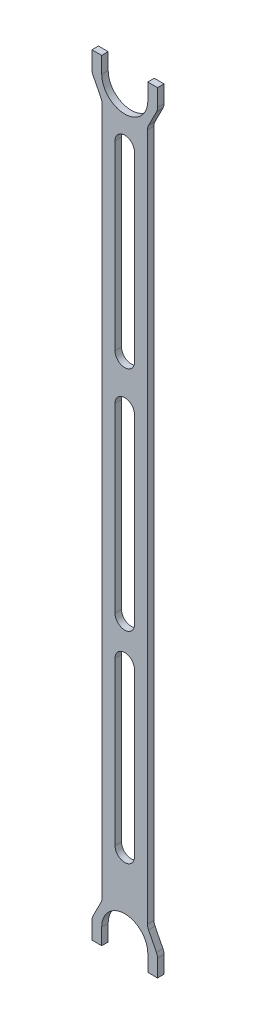
SolidWorks part; units mm, degrees
material "Thornel Mat VMA"
ref_plane "前视基准面" through (0, 0, 0) normal (0, 0, 1) x (1, 0, 0)
ref_plane "上视基准面" through (0, 0, 0) normal (0, 1, 0) x (1, 0, 0)
ref_plane "右视基准面" through (0, 0, 0) normal (1, 0, 0) x (0, 0, -1)
other "Configuration Table"
sketch "草图1" plane through (0, 0, 0) normal (0, 0, 1) x (1, 0, 0)
  line L0 (0, 106.65) -> (0, -106.65) construction
  line L1 (-7, 106.65) -> (-7, -106.65)
  line L2 (7, 106.65) -> (7, -106.65)
  line L3 (-7.1, -118.75) -> (-10.1, -118.75)
  line L4 (-10.1, -118.75) -> (-10.1, -112.75)
  line L5 (-10.1, -112.75) -> (-7, -106.65)
  line L6 (-7.1, -113.75) -> (-7.1, -118.75)
  line L7 (7.1, 113.75) -> (7.1, 118.75)
  line L8 (7.1, 118.75) -> (10.1, 118.75)
  line L9 (10.1, 118.75) -> (10.1, 112.75)
  line L10 (10.1, 112.75) -> (7, 106.65)
  line L11 (7.1, -113.75) -> (7.1, -118.75)
  line L12 (7.1, -118.75) -> (10.1, -118.75)
  line L13 (10.1, -118.75) -> (10.1, -112.75)
  line L14 (10.1, -112.75) -> (7, -106.65)
  line L15 (-10.1, 112.75) -> (-7, 106.65)
  line L16 (-10.1, 118.75) -> (-10.1, 112.75)
  line L17 (-7.1, 113.75) -> (-7.1, 118.75)
  line L18 (-7.1, 118.75) -> (-10.1, 118.75)
  line L19 (0, 98) -> (0, 42) construction
  line L20 (3, 98) -> (3, 42)
  line L21 (-3, 98) -> (-3, 42)
  line L22 (0, 28) -> (0, -28) construction
  line L23 (3, 28) -> (3, -28)
  line L24 (-3, 28) -> (-3, -28)
  line L25 (0, -40) -> (0, -90) construction
  line L26 (3, -40) -> (3, -90)
  line L27 (-3, -40) -> (-3, -90)
  circle A0 centre (0, 113.75) radius 7.1 construction
  circle A1 centre (0, -113.75) radius 7.1 construction
  arc A2 (-7.1, 113.75) -> (7.1, 113.75) centre (0, 113.75) ccw
  arc A3 (7.1, -113.75) -> (-7.1, -113.75) centre (0, -113.75) ccw
  arc A4 (3, 98) -> (-3, 98) centre (0, 98) ccw
  arc A5 (-3, 42) -> (3, 42) centre (0, 42) ccw
  arc A6 (3, 28) -> (-3, 28) centre (0, 28) ccw
  arc A7 (-3, -28) -> (3, -28) centre (0, -28) ccw
  arc A8 (3, -40) -> (-3, -40) centre (0, -40) ccw
  arc A9 (-3, -90) -> (3, -90) centre (0, -90) ccw
  point P27 (0, 70)
  point P34 (0, 0)
  point P41 (0, -65)
  dimension "D1" = 14.2
  dimension "D2" = 227.5
  dimension "D6" = 3
  dimension "D7" = 3
  dimension "D16" = 3
  dimension "D17" = 14
  dimension "D4" = 7
  dimension "D5" = 56
  dimension "D8" = 12
  dimension "D9" = 3
  dimension "D10" = 5
  dimension "D11" = 6
  dimension "D12" = 3
  dimension "D13" = 6
  dimension "D14" = 5
  dimension "D15" = 50
  dimension "D18" = 56
extrude "凸台-拉伸1" add sketch "草图1" along normal blind 2
fillet "圆角1" radius 3 8 edges at (7, -106.65, 1) (10.1, -112.75, 1) (-10.1, -112.75, 1) (-7, -106.65, 1) (-7, 106.65, 1) (-10.1, 112.75, 1) (10.1, 112.75, 1) (7, 106.65, 1)
